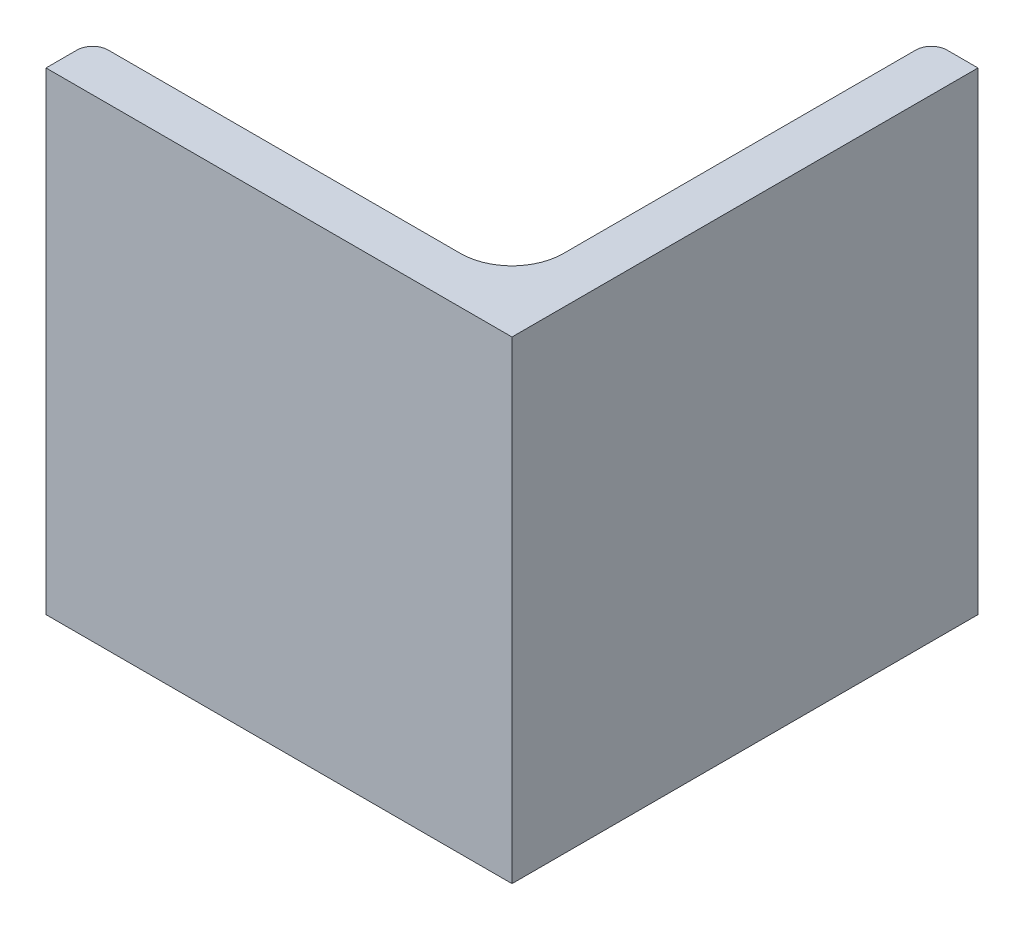
from build123d import *

# Parameters (mm, degrees)
EXTRUDE1_DEPTH = 25.4
FILLET1_R      = 5.5
FILLET2_R      = 1.67


with BuildPart() as part:
    # Sketch1 → Extrude1 (new, symmetric)
    with BuildSketch(Plane(origin=(0, 0, 0), x_dir=(1, 0, 0), z_dir=(0, 1, 0))):
        Polygon((0, -25), (0, 25), (-5, 25), (-5, -20), (-50, -20), (-50, -25), align=None)
    extrude(amount=EXTRUDE1_DEPTH, both=True)

    # Fillet1
    fillet1_edges = [part.edges().sort_by_distance(p)[0] for p in [
        (-5, 0, 20),
    ]]
    fillet(fillet1_edges, radius=FILLET1_R)

    # Fillet2
    fillet2_edges = [part.edges().sort_by_distance(p)[0] for p in [
        (-50, 0, 20),
        (-5, 0, -25),
    ]]
    fillet(fillet2_edges, radius=FILLET2_R)


solid = part.part
